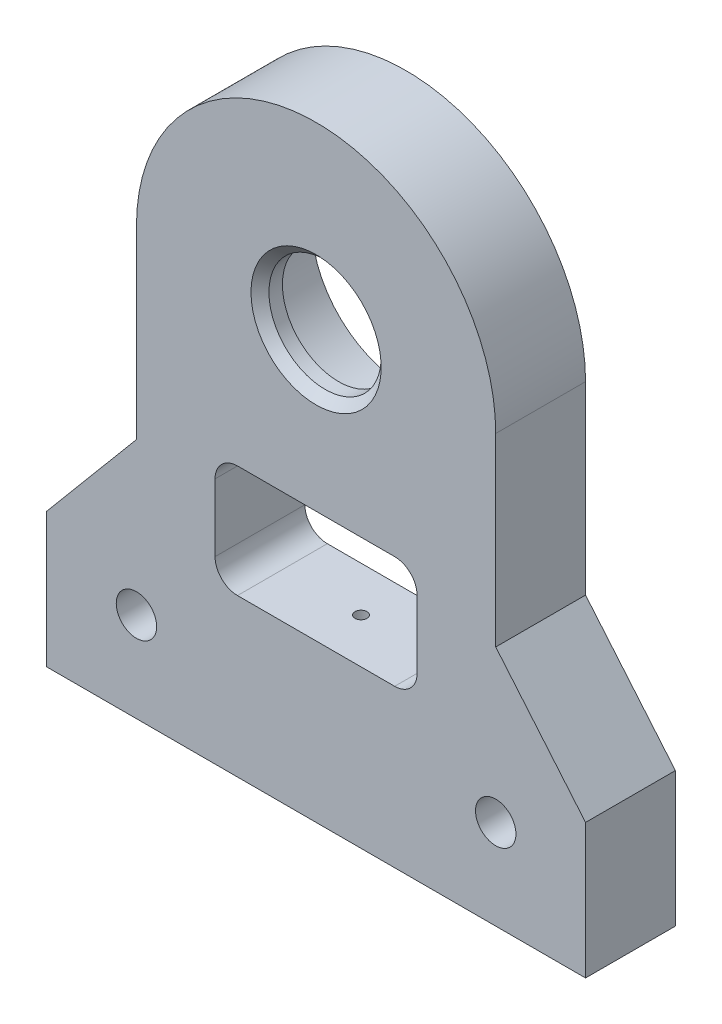
from build123d import *

# Parameters (mm, degrees)
SKETCH_1_R                = 12.5
EXTRUDE_1_DEPTH           = 10
HOLE_WIZARD_M8_1_D        = 6.8
HOLE_WIZARD_M8_1_DEPTH    = 33.75
HOLE_WIZARD_M8_1_TIP      = 2.042926105
HOLE_WIZARD_6_0_6_1_D     = 6
HOLE_WIZARD_6_0_6_1_DEPTH = 15
HOLE_WIZARD_6_0_6_1_TIP   = 1.802581857
SKETCH_6_R                = 21
CUT_EXTRUDE_1_DEPTH       = 15
CHAMFER_1_SIZE            = 2
HOLE_WIZARD_2_D           = 9
HOLE_WIZARD_2_CBORE_D     = 15
HOLE_WIZARD_2_CBORE_DEPTH = 9
CUT_EXTRUDE_2_DEPTH       = 150.080515159


with BuildPart() as part:
    # 草图1 → 凸台-拉伸1 (new, symmetric)
    with BuildSketch(Plane.XY):
        with BuildLine():
            Line((-60, 30), (-40, 53.835071852))
            Line((-40, 53.835071852), (-40, 95))
            ThreePointArc((-40, 95), (0, 135), (40, 95))
            Line((40, 95), (40, 53.835071852))
            Line((40, 53.835071852), (60, 30))
            Line((60, 30), (60, 0))
            Line((60, 0), (-60, 0))
            Line((-60, 0), (-60, 30))
        make_face()
        with Locations((0, 95)):
            Circle(SKETCH_1_R, mode=Mode.SUBTRACT)
    extrude(amount=EXTRUDE_1_DEPTH, both=True)

    # M8 螺纹孔1
    with Locations(Plane(origin=(0, 0, 0), x_dir=(-1, 0, 0), z_dir=(0, -1, 0))):
        with Locations((50, 0), (0, 0), (-50, 0)):
            Hole(HOLE_WIZARD_M8_1_D / 2, depth=HOLE_WIZARD_M8_1_DEPTH)
            with Locations((0, 0, -(HOLE_WIZARD_M8_1_DEPTH + HOLE_WIZARD_M8_1_TIP / 2))):  # 118° drill point
                Cone(0, HOLE_WIZARD_M8_1_D / 2, HOLE_WIZARD_M8_1_TIP, mode=Mode.SUBTRACT)

    # Ø6.0 (6) 直径孔1
    with Locations(Plane(origin=(0, 0, 0), x_dir=(-1, 0, 0), z_dir=(0, -1, 0))):
        with Locations((-35, 0), (35, 0)):
            Hole(HOLE_WIZARD_6_0_6_1_D / 2, depth=HOLE_WIZARD_6_0_6_1_DEPTH)
            with Locations((0, 0, -(HOLE_WIZARD_6_0_6_1_DEPTH + HOLE_WIZARD_6_0_6_1_TIP / 2))):  # 118° drill point
                Cone(0, HOLE_WIZARD_6_0_6_1_D / 2, HOLE_WIZARD_6_0_6_1_TIP, mode=Mode.SUBTRACT)

    # 草图6 → 切除-拉伸1 (cut)
    with BuildSketch(Plane.XY.offset(-10)):
        with Locations((0, 95)):
            Circle(SKETCH_6_R)
    extrude(amount=CUT_EXTRUDE_1_DEPTH, mode=Mode.SUBTRACT)

    # 倒角1
    chamfer_1_edges = [part.edges().sort_by_distance(p)[0] for p in [
        (-12.5, 95, 10),
    ]]
    chamfer(chamfer_1_edges, length=CHAMFER_1_SIZE)

    # 打孔尺寸(%根据)内六角圆柱头螺钉的类型2 (through all)
    with Locations(Plane(origin=(0, 0, -10), x_dir=(-1, 0, 0), z_dir=(0, 0, -1))):
        with Locations((-40, 20), (40, 20)):
            CounterBoreHole(HOLE_WIZARD_2_D / 2, HOLE_WIZARD_2_CBORE_D / 2, HOLE_WIZARD_2_CBORE_DEPTH)

    # 草图13 → 切除-拉伸2 (cut, through all)
    with BuildSketch(Plane(origin=(0, 0, -10), x_dir=(-1, 0, 0), z_dir=(0, 0, -1))):
        with BuildLine():
            Line((17.5, 60), (-17.5, 60))
            ThreePointArc((-17.5, 60), (-21.035533906, 58.535533906), (-22.5, 55))
            Line((-22.5, 55), (-22.5, 40))
            ThreePointArc((-22.5, 40), (-21.035533906, 36.464466094), (-17.5, 35))
            Line((-17.5, 35), (17.5, 35))
            ThreePointArc((17.5, 35), (21.035533906, 36.464466094), (22.5, 40))
            Line((22.5, 40), (22.5, 55))
            ThreePointArc((22.5, 55), (21.035533906, 58.535533906), (17.5, 60))
        make_face()
    extrude(amount=-CUT_EXTRUDE_2_DEPTH, mode=Mode.SUBTRACT)


solid = part.part
